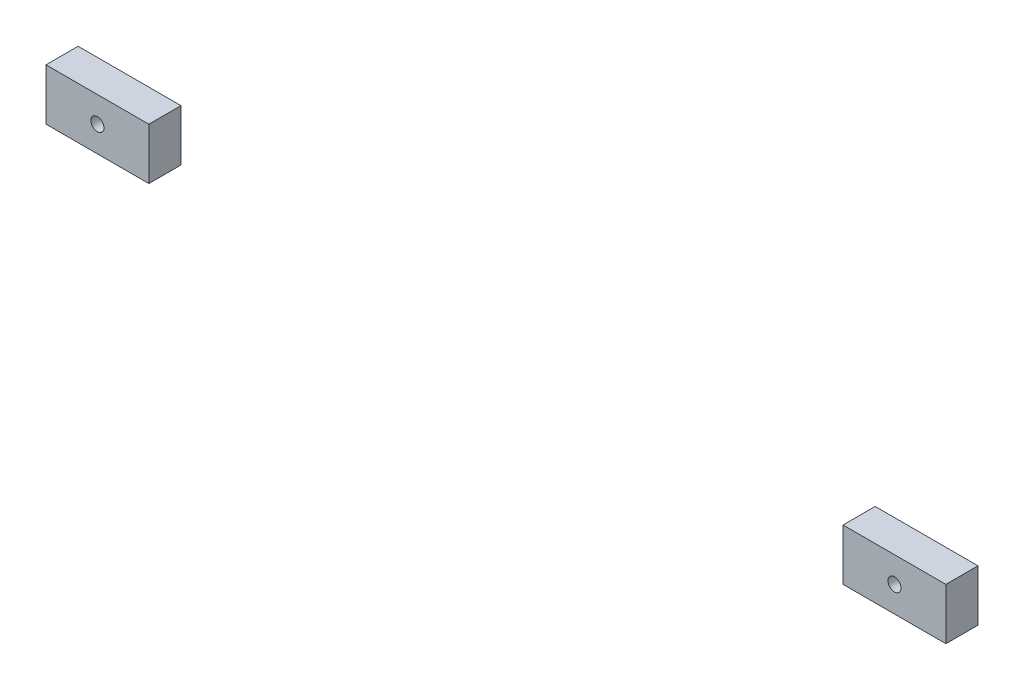
SolidWorks part; units mm, degrees
material "Plain carbon steel"
ref_plane "Front Plane" through (0, 0, 0) normal (0, 0, 1) x (1, 0, 0)
ref_plane "Top Plane" through (0, 0, 0) normal (0, 1, 0) x (1, 0, 0)
ref_plane "Right Plane" through (0, 0, 0) normal (1, 0, 0) x (0, 0, -1)
sketch "Sketch1" plane through (0, 0, 0) normal (0, 0, 1) x (1, 0, 0)
  line L1 (0, 0) -> (80, 0)
  line L2 (0, 0) -> (0, -40)
  line L3 (0, -40) -> (80, -40)
  line L4 (80, 0) -> (80, -40)
  line L5 (620, 0) -> (700, 0)
  line L6 (620, 0) -> (620, -40)
  line L7 (620, -40) -> (700, -40)
  line L8 (700, 0) -> (700, -40)
  dimension "D1" = 40
  dimension "D2" = 80
  dimension "D3" = 620
extrude "Boss-Extrude1" add sketch "Sketch1" along normal blind 25
hole_wizard "M12 Tapped Hole1" positions "Sketch2" profile "Sketch3" tap size "M12" standard "GB" end condition through all
sketch "Sketch2" plane through (0, 0, 25) normal (0, 0, 1) x (1, 0, 0)
  line L0 (40, -40) -> (40, -20) construction
  line L1 (0, -40) -> (80, -40) construction
  line L3 (0, -20) -> (40, -20) construction
  line L4 (0, 0) -> (0, -40) construction
  line L9 (660, -40) -> (660, -20) construction
  line L10 (620, -40) -> (700, -40) construction
  point P0 (40, -20)
  point P2 (660, -20)
sketch "Sketch3" plane through (40, -20, 25) normal (1, 0, 0) x (0, -1, 0)
  line L0 (0, 0) -> (0, 25)
  line L1 (0, 25) -> (5.1, 25)
  line L2 (5.1, 25) -> (5.1, 0)
  line L5 (5.1, 0) -> (0, 0)
  line L11 (0, -6.35) -> (0, 107.95) construction
  dimension "通孔螺纹孔钻头直径" = 10.2
  dimension "通孔螺纹孔钻头深度" = 25
cosmetic thread "Cosmetic Thread1" parameters "D1"=16, "D2"=11.2
cosmetic thread "Cosmetic Thread2" parameters "D1"=16, "D2"=11.2
